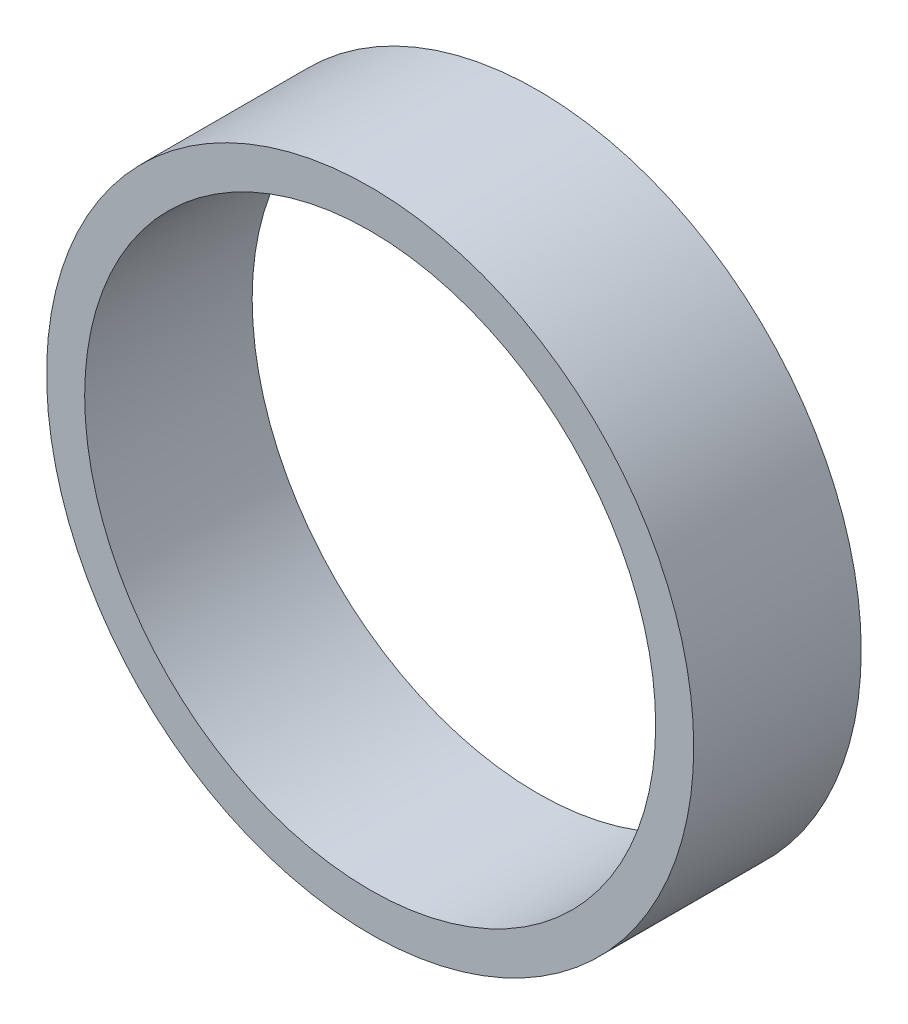
SolidWorks part; units mm, degrees
ref_plane "前视基准面" through (0, 0, 0) normal (0, 0, 1) x (1, 0, 0)
ref_plane "上视基准面" through (0, 0, 0) normal (0, 1, 0) x (1, 0, 0)
ref_plane "右视基准面" through (0, 0, 0) normal (1, 0, 0) x (0, 0, -1)
other "Configuration Table"
sketch "草图1" plane through (0, 0, 0) normal (0, 0, 1) x (1, 0, 0)
  circle A0 centre (0, 0) radius 37.5
  circle A1 centre (0, 0) radius 42.5
  dimension "D1" = 85
  dimension "D2" = 75
extrude "凸台-拉伸1" add sketch "草图1" along normal blind 22
